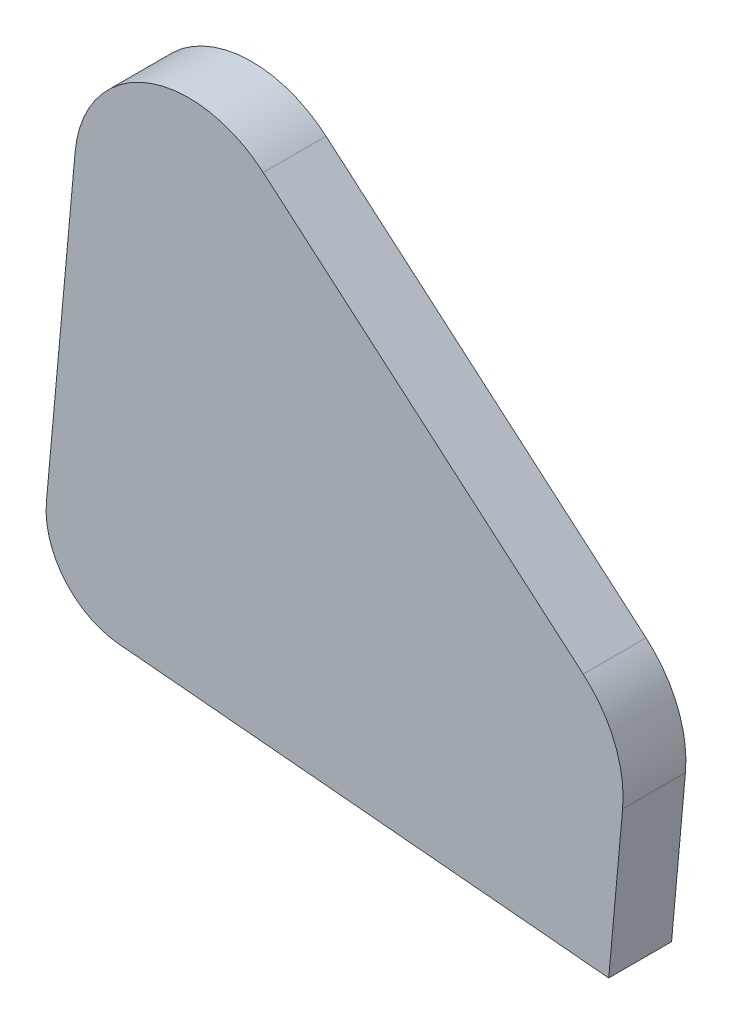
SolidWorks part; units mm, degrees
material "AISI 304"
ref_plane "Front Plane" through (0, 0, 0) normal (0, 0, 1) x (1, 0, 0)
ref_plane "Top Plane" through (0, 0, 0) normal (0, 1, 0) x (1, 0, 0)
ref_plane "Right Plane" through (0, 0, 0) normal (1, 0, 0) x (0, 0, -1)
other "Configuration Table"
sketch "Sketch1" plane through (0, 0, 0) normal (0, 0, 1) x (1, 0, 0)
  line L4 (-199.1866, 18.0191) -> (-249.4306, -537.3866)
  line L5 (-122.6134, -689.4306) -> (735.0597, -767.0188)
  line L8 (759.3562, -498.4418) -> (735.0597, -767.0188)
  line L9 (130.2016, 151.8142) -> (690.3711, -328.6085)
  arc A0 (130.2016, 151.8142) -> (-199.1866, 18.0191) centre (0, 0) ccw
  arc A3 (-249.4306, -537.3866) -> (-122.6134, -689.4306) centre (-110, -550) ccw
  arc A7 (759.3562, -498.4418) -> (690.3711, -328.6085) centre (560.1695, -480.4227) ccw
  dimension "D1" = 400
  dimension "D2" = 400
  dimension "D4" = 280
  dimension "D5" = 110
  dimension "D6" = 550
extrude "Boss-Extrude2" add sketch "Sketch1" along normal blind 110
shell "Shell2" thickness 3
